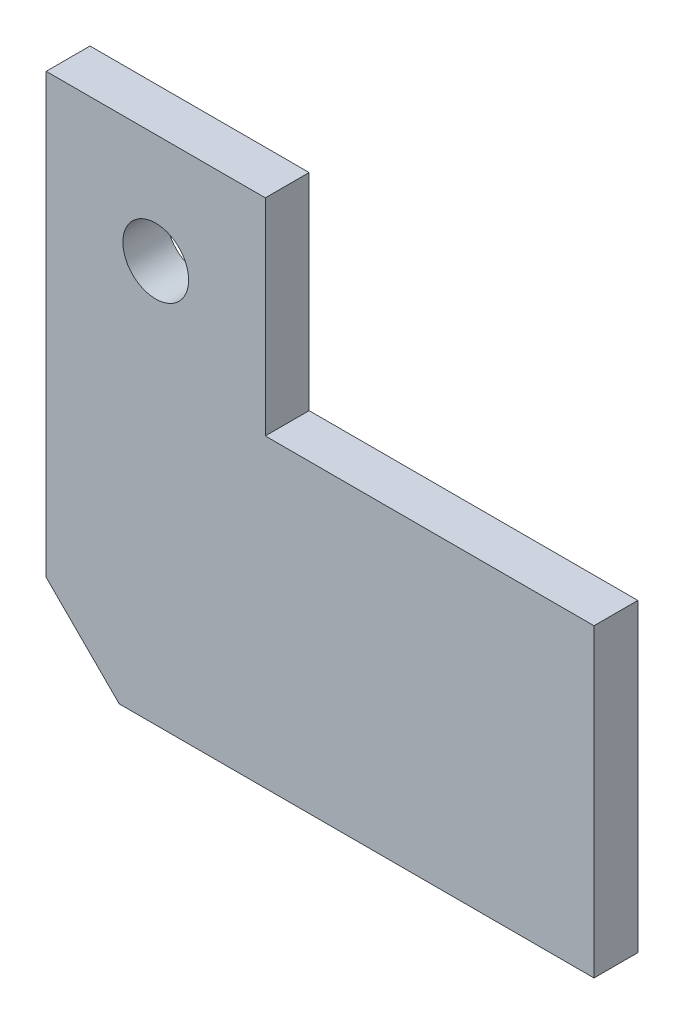
from build123d import *

# Parameters (mm, degrees)
BOSS_EXTRUDE1_DEPTH = 6
CUT_EXTRUDE1_REACH  = 68.303
SKETCH2_R           = 4.5
CHAMFER1_SIZE       = 10


with BuildPart() as part:
    # Sketch1 → Boss-Extrude1 (new body)
    with BuildSketch(Plane.XY):
        Polygon((-33.521587555, -18.6224812), (-33.521587555, 51.3775188), (-3.521587555, 51.3775188), (-3.521587555, 23.144505274), (41.478412445, 23.144505274), (41.478412445, -18.6224812), align=None)
    extrude(amount=BOSS_EXTRUDE1_DEPTH)

    # Sketch2 → Cut-Extrude1 (cut, up to next)
    with BuildSketch(Plane.XY.offset(6), mode=Mode.PRIVATE) as cut_extrude1_sk1:
        with Locations((-18.521587555, 36.3775188)):
            Circle(SKETCH2_R)
    cut_extrude1_tool1 = extrude(cut_extrude1_sk1.sketch, amount=-CUT_EXTRUDE1_REACH, mode=Mode.PRIVATE) & part.part
    add(cut_extrude1_tool1.solids().sort_by_distance((-18.521588, 36.377519, 6))[0], mode=Mode.SUBTRACT)

    # Chamfer1
    chamfer1_edges = [part.edges().sort_by_distance(p)[0] for p in [
        (-33.521587555, -18.6224812, 3),
    ]]
    chamfer(chamfer1_edges, length=CHAMFER1_SIZE)


solid = part.part
